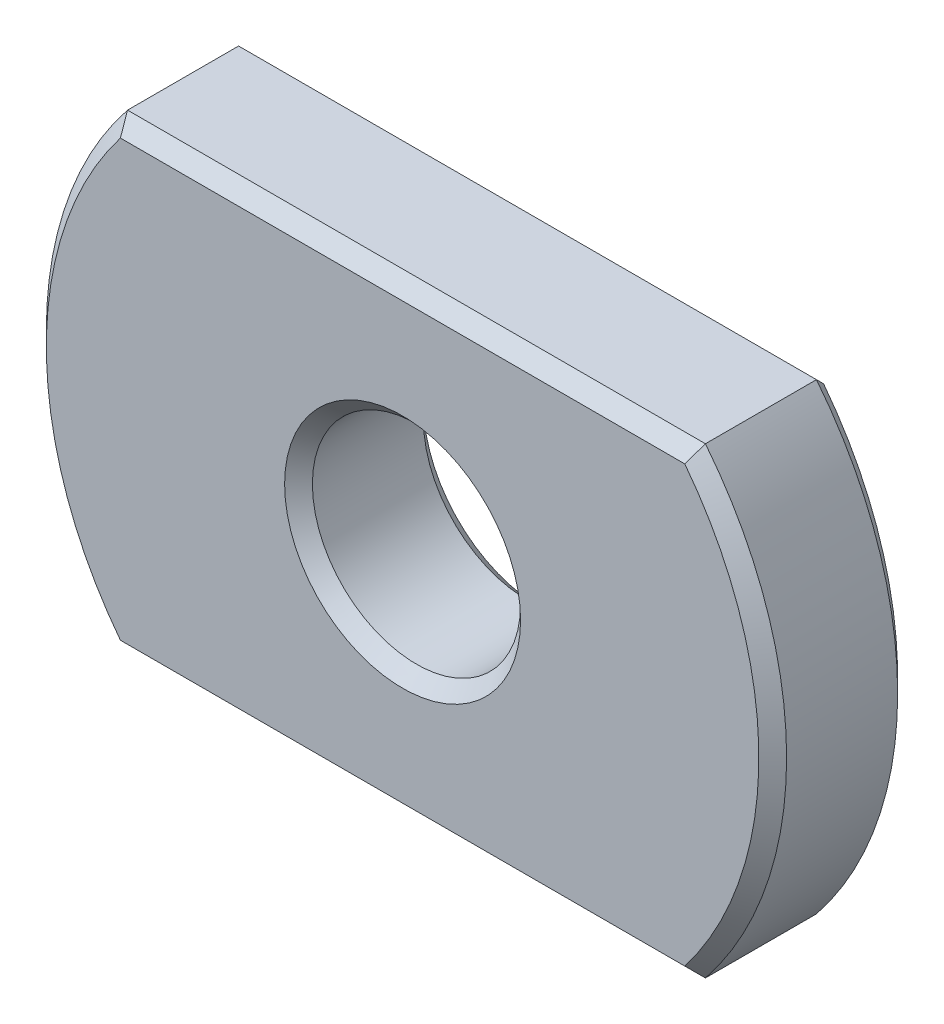
from build123d import *

# Parameters (mm, degrees)
SKETCH1_R           = 8
SKETCH1_R_2         = 2.25
BOSS_EXTRUDE1_DEPTH = 1.5
SKETCH2_OUTSIDE_W   = 22.566
SKETCH2_OUTSIDE_H   = 22.566
SKETCH2_OUTSIDE_W_2 = 20
SKETCH2_OUTSIDE_H_2 = 10
CUT_EXTRUDE1_DEPTH  = 12.704699911
CHAMFER1_SIZE       = 0.3


with BuildPart() as part:
    # Sketch1 → Boss-Extrude1 (new, symmetric)
    with BuildSketch(Plane.XY):
        Circle(SKETCH1_R)
        Circle(SKETCH1_R_2, mode=Mode.SUBTRACT)
    extrude(amount=BOSS_EXTRUDE1_DEPTH, both=True)

    # Sketch2 outside → Cut-Extrude1 (cut, through all)
    with BuildSketch(Plane.XY.offset(1.5)):
        Rectangle(SKETCH2_OUTSIDE_W, SKETCH2_OUTSIDE_H)
        Rectangle(SKETCH2_OUTSIDE_W_2, SKETCH2_OUTSIDE_H_2, mode=Mode.SUBTRACT)
    extrude(amount=-CUT_EXTRUDE1_DEPTH, mode=Mode.SUBTRACT)

    # Chamfer1
    chamfer1_edges = [part.edges().sort_by_distance(p)[0] for p in [
        (8, 0, 1.5),
        (-8, 0, -1.5),
        (8, 0, -1.5),
        (0, 5, -1.5),
        (0, -5, -1.5),
        (0, -5, 1.5),
        (0, 5, 1.5),
        (-2.25, 0, -1.5),
        (-2.25, 0, 1.5),
        (-8, 0, 1.5),
    ]]
    chamfer(chamfer1_edges, length=CHAMFER1_SIZE)


solid = part.part
